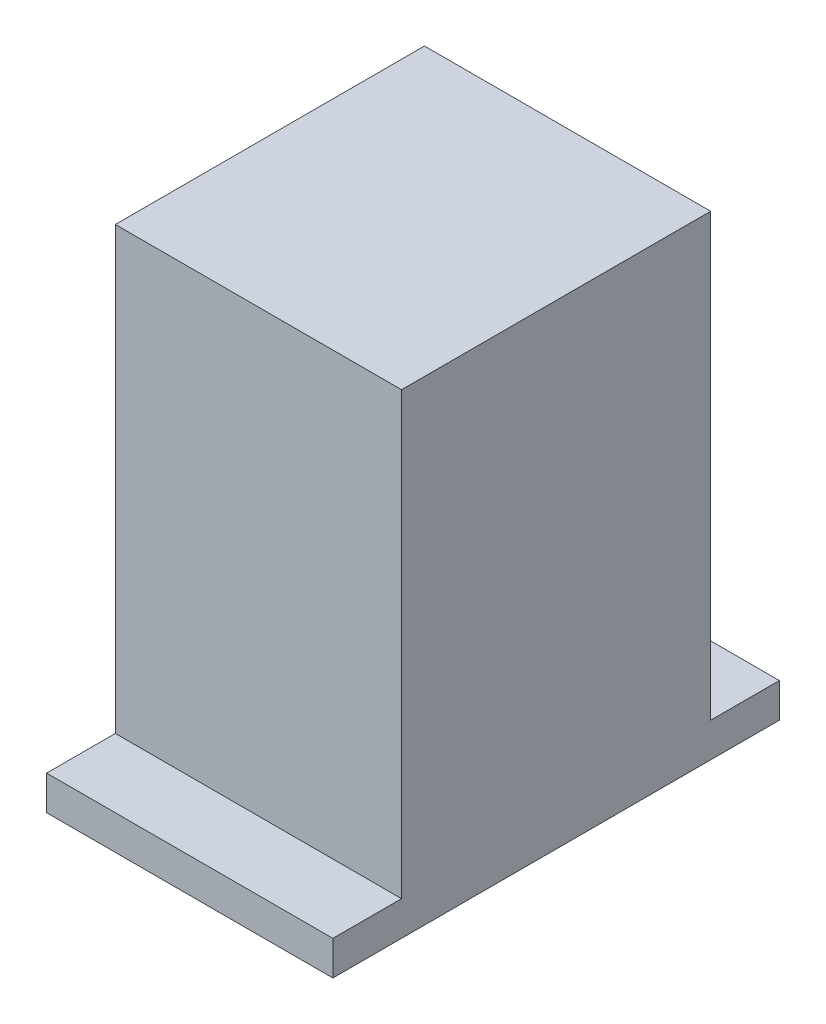
from build123d import *

# Parameters (mm, degrees)
SKETCH1_W           = 50
SKETCH1_H           = 83
BOSS_EXTRUDE1_DEPTH = 39
SKETCH2_W           = 12
SKETCH2_H           = 77
CUT_EXTRUDE1_DEPTH  = 76.784233189


with BuildPart() as part:
    # Sketch1 → Boss-Extrude1 (new, symmetric)
    with BuildSketch(Plane.XY):
        Rectangle(SKETCH1_W, SKETCH1_H)
    extrude(amount=BOSS_EXTRUDE1_DEPTH, both=True)

    # Sketch2 → Cut-Extrude1 (cut, through all)
    with BuildSketch(Plane.ZY.offset(25)):
        with Locations((-33, 3)):
            Rectangle(SKETCH2_W, SKETCH2_H)
        with Locations((33, 3)):
            Rectangle(SKETCH2_W, SKETCH2_H)
    extrude(amount=-CUT_EXTRUDE1_DEPTH, mode=Mode.SUBTRACT)


solid = part.part
